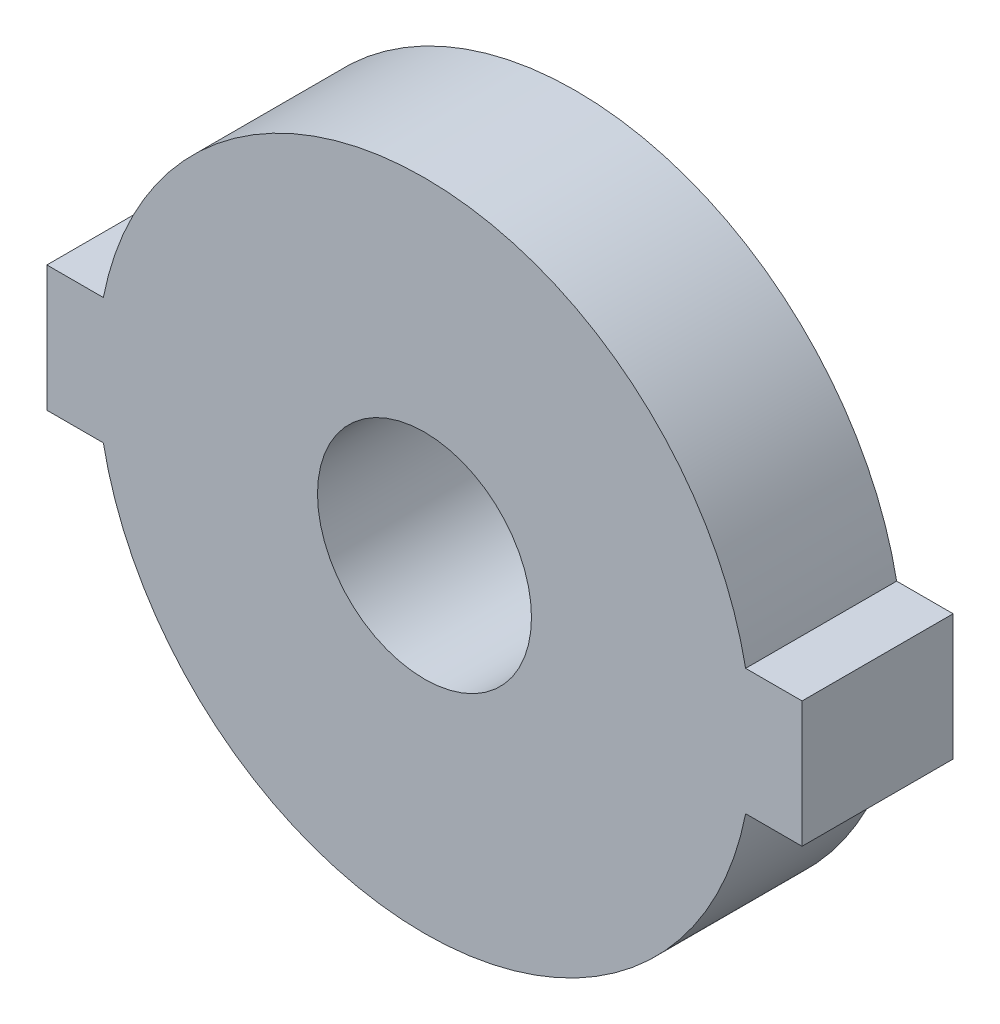
SolidWorks part; units mm, degrees
ref_plane "Front Plane" through (0, 0, 0) normal (0, 0, 1) x (1, 0, 0)
ref_plane "Top Plane" through (0, 0, 0) normal (0, 1, 0) x (1, 0, 0)
ref_plane "Right Plane" through (0, 0, 0) normal (1, 0, 0) x (0, 0, -1)
other "Configuration Table"
ref_plane "Plane1" through (0, 0, 6) normal (0, 0, 1) x (1, 0, 0)
sketch "Sketch1" plane through (0, 0, 6) normal (0, 0, 1) x (1, 0, 0)
  line L0 (-12.7574, 2.5) -> (-15, 2.5)
  line L1 (-15, 2.5) -> (-15, -2.5)
  line L2 (-15, -2.5) -> (-12.7574, -2.5)
  line L3 (12.7574, -2.5) -> (15, -2.5)
  line L4 (15, -2.5) -> (15, 2.5)
  line L5 (15, 2.5) -> (12.7574, 2.5)
  circle A0 centre (0, 0) radius 4.25
  arc A1 (12.7574, 2.5) -> (-12.7574, 2.5) centre (0, 0) ccw
  arc A2 (-12.7574, -2.5) -> (12.7574, -2.5) centre (0, 0) ccw
extrude "Boss-Extrude1" add sketch "Sketch1" against normal blind 6
